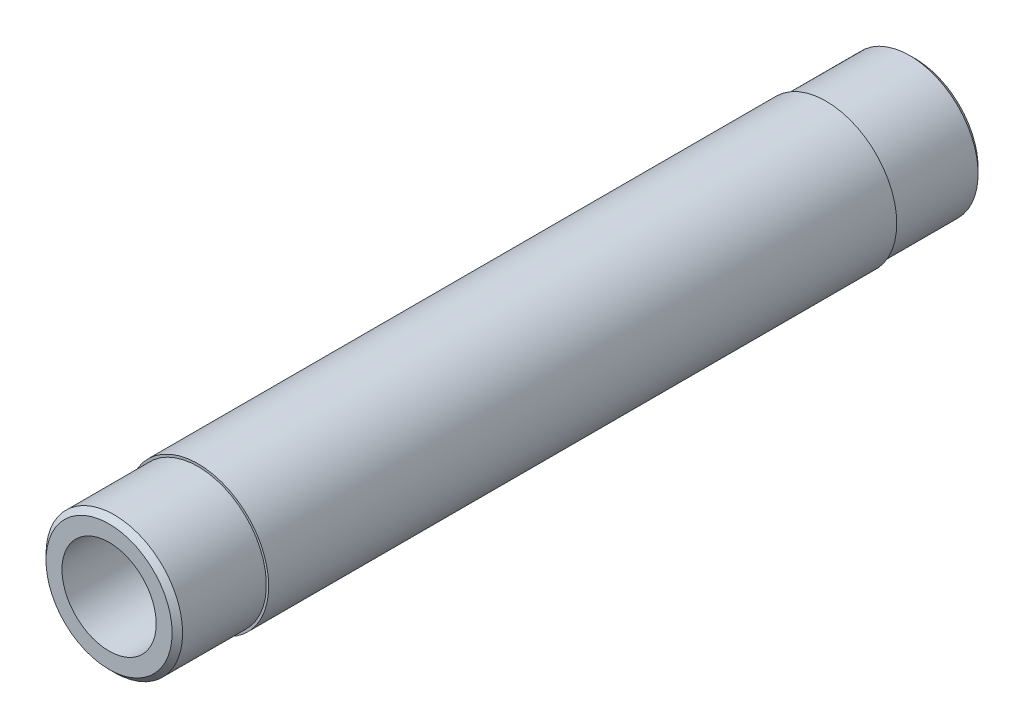
from build123d import *

# Parameters (mm, degrees)
SKETCH_1_R          = 13.5
EXTRUDE_1_DEPTH     = 60
SKETCH_4_R          = 13.05
EXTRUDE_3_DEPTH     = 17
CUT_EXTRUDE_2_REACH = 157.179
SKETCH_5_R          = 9
CHAMFER_1_SIZE      = 1


with BuildPart() as part:
    # 草图1 → 凸台-拉伸1 (new, symmetric)
    with BuildSketch(Plane.XY):
        Circle(SKETCH_1_R)
    extrude(amount=EXTRUDE_1_DEPTH, both=True)

    # 草图4 → 凸台-拉伸3 (add)
    with BuildSketch(Plane(origin=(0, 0, -60), x_dir=(-1, 0, 0), z_dir=(0, 0, -1))):
        Circle(SKETCH_4_R)
    extrude_3 = extrude(amount=EXTRUDE_3_DEPTH)

    # 镜向1: 凸台-拉伸3 across plane
    add(extrude_3.mirror(Plane.XY))

    # 草图5 → 切除-拉伸2 (cut, up to next)
    with BuildSketch(Plane(origin=(0, 0, -77), x_dir=(-1, 0, 0), z_dir=(0, 0, -1)), mode=Mode.PRIVATE) as cut_extrude_2_sk1:
        Circle(SKETCH_5_R)
    cut_extrude_2_tool1 = extrude(cut_extrude_2_sk1.sketch, amount=-CUT_EXTRUDE_2_REACH, mode=Mode.PRIVATE) & part.part
    add(cut_extrude_2_tool1.solids().sort_by_distance((0, 0, -77))[0], mode=Mode.SUBTRACT)

    # 倒角1
    chamfer_1_edges = [part.edges().sort_by_distance(p)[0] for p in [
        (13.05, 0, 77),
        (13.05, 0, -77),
    ]]
    chamfer(chamfer_1_edges, length=CHAMFER_1_SIZE)


solid = part.part
